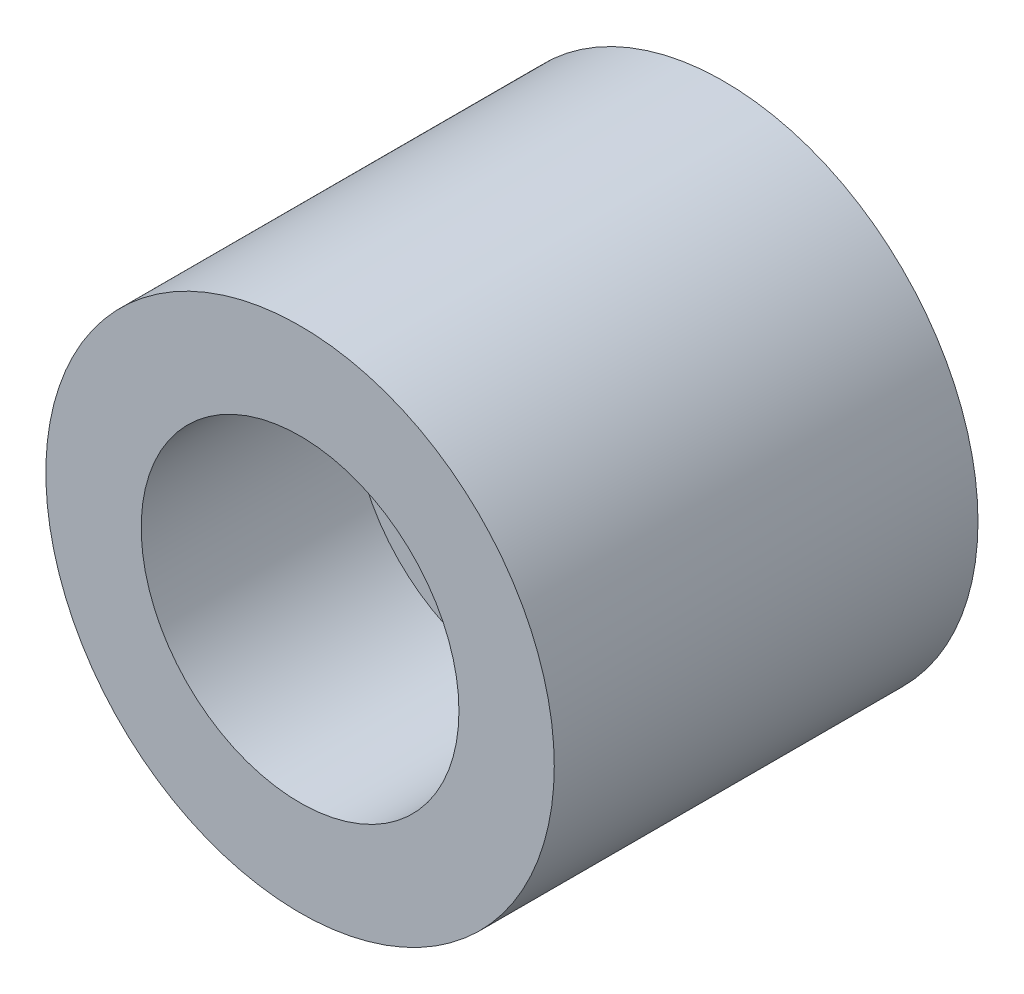
from build123d import *

# Parameters (mm, degrees)
SKETCH_1_R                = 6
EXTRUDE_1_DEPTH           = 10
HOLE_WIZARD_1_D           = 4.5
HOLE_WIZARD_1_CBORE_D     = 7.5
HOLE_WIZARD_1_CBORE_DEPTH = 5


with BuildPart() as part:
    # 草图1 → 凸台-拉伸1 (new body)
    with BuildSketch(Plane.XY):
        Circle(SKETCH_1_R)
    extrude(amount=EXTRUDE_1_DEPTH)

    # 打孔尺寸(%根据)内六角圆柱头螺钉的类型1 (through all)
    with Locations(Plane.XY.offset(10)):
        with Locations((0, 0)):
            CounterBoreHole(HOLE_WIZARD_1_D / 2, HOLE_WIZARD_1_CBORE_D / 2, HOLE_WIZARD_1_CBORE_DEPTH)


solid = part.part
